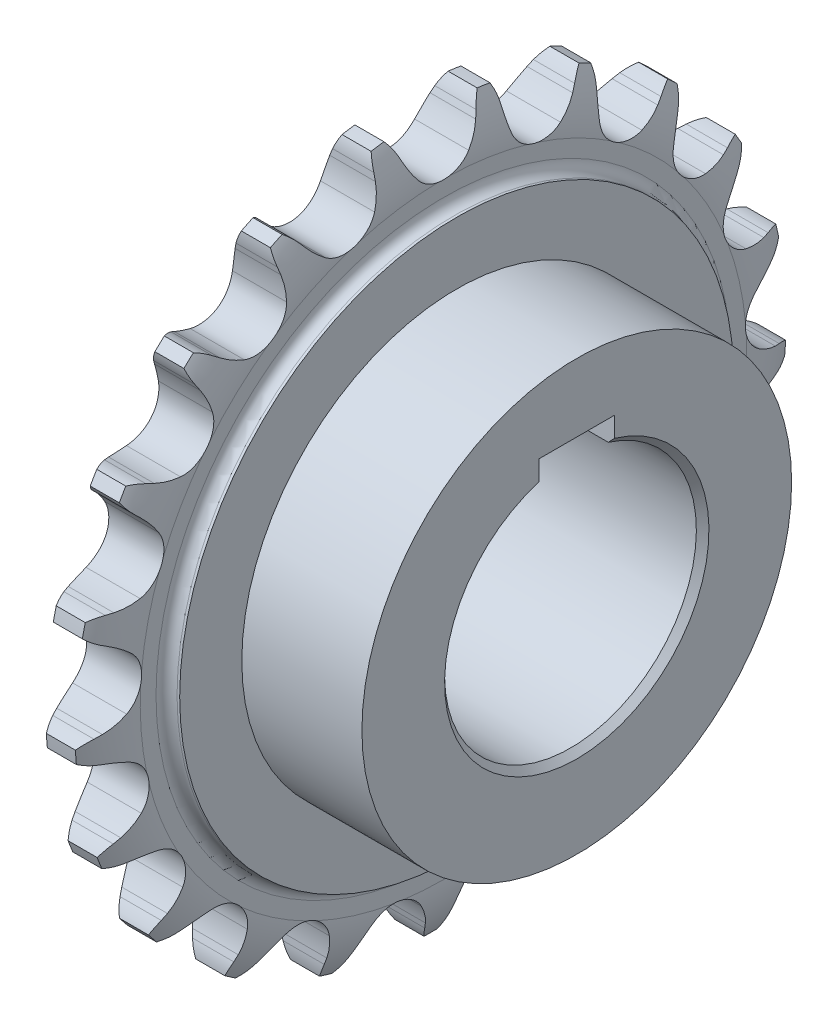
SolidWorks part; units mm, degrees
ref_plane "前视基准面" through (0, 0, 0) normal (0, 0, 1) x (1, 0, 0)
ref_plane "上视基准面" through (0, 0, 0) normal (0, 1, 0) x (1, 0, 0)
ref_plane "右视基准面" through (0, 0, 0) normal (1, 0, 0) x (0, 0, -1)
sketch "草图1" plane through (0, 0, 0) normal (0, 0, 1) x (1, 0, 0)
  line L0 (-7.9375, 0) -> (7.9375, 0) construction
  line L1 (-6.4594, 20) -> (-6.4594, 44)
  line L2 (-6.4594, 44) -> (-6.0417, 44)
  line L3 (-4.371, 45.6707) -> (-4.371, 48.1767)
  line L4 (-2.3072, 56.5) -> (2.3072, 56.5)
  line L5 (4.371, 48.1767) -> (4.371, 45.6707)
  line L6 (6.0417, 44) -> (6.4594, 44)
  line L7 (6.4594, 44) -> (6.4594, 20)
  line L8 (6.4594, 20) -> (-6.4594, 20)
  line L9 (0, 0) -> (0, 56.5) construction
  line L10 (-3.6982, 53.2567) -> (3.6982, 53.2567) construction
  line L11 (-3.6982, -53.2567) -> (3.6982, -53.2567) construction
  line L12 (7.9375, 0) -> (28.9375, 0) construction
  line L13 (-4.371, 48.1767) -> (3.7984, 48.1767) construction
  line L14 (-4.371, -48.1767) -> (3.7984, -48.1767) construction
  line L15 (28.9375, 0) -> (39.0975, 0) construction
  line L16 (39.0975, 0) -> (54.1875, 0) construction
  line L17 (54.1875, 0) -> (63.5875, 0) construction
  line L18 (63.5875, 0) -> (81.6975, 0) construction
  arc A0 (-2.3072, 56.5) -> (-4.371, 48.1767) centre (11.4966, 48.6598) ccw
  arc A1 (2.3072, 56.5) -> (4.371, 48.1767) centre (-11.4966, 48.6598) cw
  arc A2 (4.371, 45.6707) -> (6.0417, 44) centre (6.0417, 45.6707) ccw
  arc A3 (-6.0417, 44) -> (-4.371, 45.6707) centre (-6.0417, 45.6707) ccw
  point P30 (4.371, 44)
  point P33 (-4.371, 44)
  dimension "D1" = 4.1767
  dimension "rx" = 15.875
  dimension "D3" = 1.6707
  dimension "d" = 106.5134
  dimension "p" = 15.875
  dimension "z" = 21
  dimension "da" = 113
  dimension "df" = 96.3534
  dimension "dr" = 10.16
  dimension "dk" = 40
  dimension "dg" = 88
  dimension "h" = 15.09
  dimension "bf1" = 8.742
  dimension "b1" = 9.4
  dimension "ba" = 2.0638
  dimension "D2" = 2.0884
  dimension "pt" = 18.11
revolve "旋转1" add sketch "草图1" angle 360 about L0
sketch "草图2" plane through (0, 0, 0) normal (1, 0, 0) x (0, 0, -1)
  line L0 (0, 0) -> (0, 56.5) construction
  line L1 (0, 0) -> (-8.4209, 55.8689) construction
  line L2 (0, 0) -> (-16.6537, 53.9899) construction
  line L3 (4.0704, 50.0929) -> (10.2701, 45.274) construction
  line L4 (5.8527, 53.1564) -> (-6.4174, 58.2448) construction
  line L5 (0, 0) -> (8.4209, 55.8689) construction
  line L6 (5.8527, 53.1564) -> (6.2493, 54.1127)
  line L7 (-5.8527, 53.1564) -> (-6.2493, 54.1127)
  circle A0 centre (0, 0) radius 56.5 construction
  arc A1 (4.0704, 50.0929) -> (-4.0704, 50.0929) centre (0, 53.2567) cw
  arc A2 (4.0704, 50.0929) -> (5.8527, 53.1564) centre (-6.4174, 58.2448) ccw
  arc A3 (7.3999, 56.0133) -> (6.2493, 54.1127) centre (13.0605, 51.2882) ccw
  arc A4 (-4.0704, 50.0929) -> (-5.8527, 53.1564) centre (6.4174, 58.2448) cw
  arc A5 (-7.3999, 56.0133) -> (-6.2493, 54.1127) centre (-13.0605, 51.2882) cw
  arc A7 (7.3999, 56.0133) -> (-7.3999, 56.0133) centre (0, 0) ccw
  dimension "r1" = 5.1554
  dimension "r3" = 7.3736
  dimension "D1" = 17.143
  dimension "D2" = 8.571
  dimension "α/2" = 52.143
  dimension "M" = 6.4174
  dimension "T" = 4.9881
  dimension "β" = 15.333
  dimension "γ/2" = 13.952
  dimension "bc" = 1.0353
extrude "切除-拉伸1" cut sketch "草图2" against normal mid plane 12.9187
pattern_circular "阵列(圆周)1" count 21 over 360 about axis through (0, 0, 0) along (1, 0, 0) of "切除-拉伸1"
sketch "草图3" plane through (0, 0, 0) normal (0, 0, 1) x (1, 0, 0)
  line L0 (6.4594, 20) -> (25.5406, 20)
  line L3 (25.5406, 20) -> (25.5406, 34.1318)
  line L4 (25.5406, 34.1318) -> (6.4594, 34.1318)
  line L5 (6.4594, 34.1318) -> (6.4594, 20)
  line L6 (0, 0) -> (6.4, 0) construction
  line L8 (-6.4594, 44) -> (-6.4594, -44) construction
  dimension "h" = 14.1318
  dimension "K" = 6.4
  dimension "L" = 32
revolve "旋转2" add sketch "草图3" angle 360 about L6
sketch "草图4" plane through (-6.4594, 0, 0) normal (-1, 0, 0) x (0, 0, 1)
  line L1 (-6, 19.0788) -> (6, 19.0788)
  line L2 (-6, 19.0788) -> (-6, 23.3)
  line L3 (-6, 23.3) -> (6, 23.3)
  line L4 (6, 19.0788) -> (6, 23.3)
  circle A0 centre (0, 0) radius 20 construction
  point P6 (2.7, 23.3)
  dimension "D1" = 23.3
  dimension "键槽宽度" = 12
  dimension "t1" = 3.3
extrude "切除-拉伸2" cut sketch "草图4" against normal through all
chamfer "倒角1" distance 1 angle 45 1 edges at (-6.4594, -20, 0)
chamfer "倒角3" distance 1 angle 45 1 edges at (25.5406, -20, 0)
